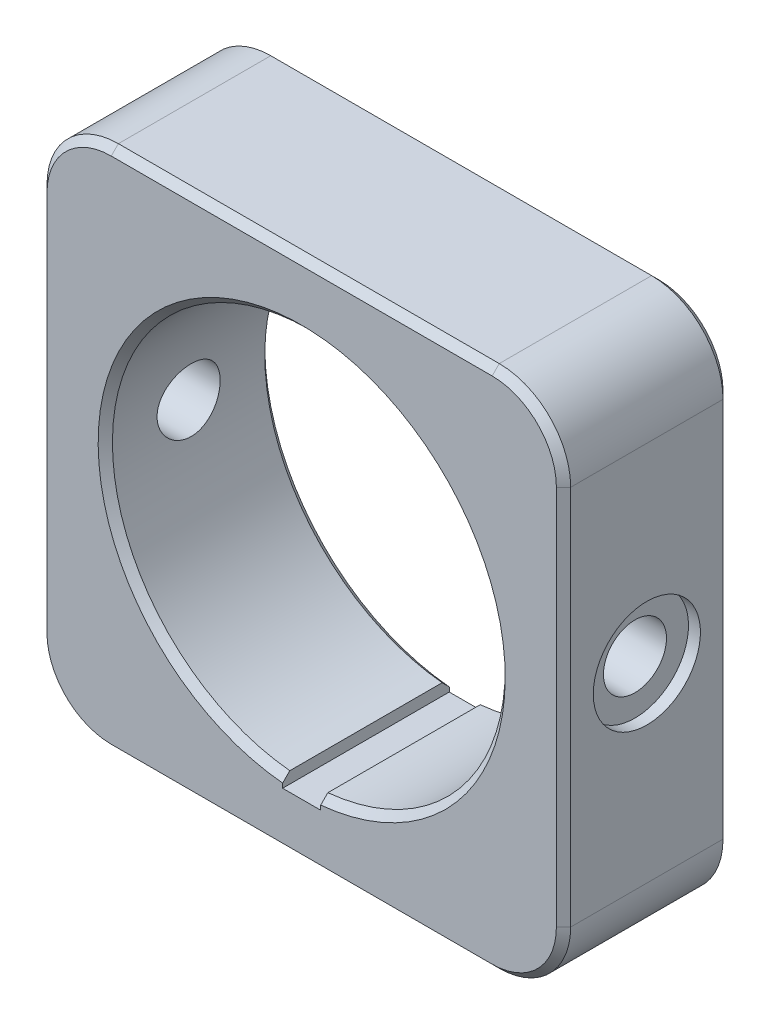
from build123d import *

# Parameters (mm, degrees)
SKETCH1_W           = 220
SKETCH1_H           = 220
BOSS_EXTRUDE1_DEPTH = 70
SKETCH2_R           = 82.5
CUT_EXTRUDE1_DEPTH  = 171.587221092
M30_TAPPED_HOLE1_D  = 26.5
SKETCH7_R           = 22.5
CUT_EXTRUDE3_DEPTH  = 5
FILLET1_R           = 30
CHAMFER1_SIZE       = 3
SKETCH8_W           = 16
SKETCH8_H           = 87
CUT_EXTRUDE4_DEPTH  = 171.587221092


with BuildPart() as part:
    # Sketch1 → Boss-Extrude1 (new body)
    with BuildSketch(Plane.XY):
        Rectangle(SKETCH1_W, SKETCH1_H)
    extrude(amount=BOSS_EXTRUDE1_DEPTH)

    # Sketch2 → Cut-Extrude1 (cut, through all)
    with BuildSketch(Plane.XY.offset(70)):
        Circle(SKETCH2_R)
    extrude(amount=-CUT_EXTRUDE1_DEPTH, mode=Mode.SUBTRACT)

    # M30 Tapped Hole1 (through all)
    with Locations(Plane(origin=(110, 0, 0), x_dir=(0, 0, -1), z_dir=(1, 0, 0))):
        with Locations((-35, 0)):
            Hole(M30_TAPPED_HOLE1_D / 2)

    # Sketch7 → Cut-Extrude3 (cut)
    with BuildSketch(Plane.ZY.offset(110)):
        with Locations((35, 0)):
            Circle(SKETCH7_R)
    cut_extrude3 = extrude(amount=-CUT_EXTRUDE3_DEPTH, mode=Mode.SUBTRACT)

    # Mirror1: Cut-Extrude3 across plane
    add(cut_extrude3.mirror(Plane(origin=(0, 0, 0), x_dir=(0, 0, 1), z_dir=(1, 0, 0))), mode=Mode.SUBTRACT)

    # Fillet1
    fillet1_edges = [part.edges().sort_by_distance(p)[0] for p in [
        (-110, 110, 35),
        (110, 110, 35),
        (110, -110, 35),
        (-110, -110, 35),
    ]]
    fillet(fillet1_edges, radius=FILLET1_R)

    # Chamfer1
    chamfer1_edges = [part.edges().sort_by_distance(p)[0] for p in [
        (-82.5, 0, 0),
        (-82.5, 0, 70),
        (0, 110, 0),
        (0, 110, 70),
        (-110, 0, 0),
        (110, 0, 0),
        (0, -110, 0),
        (-101.213203436, 101.213203436, 0),
        (-101.213203436, -101.213203436, 0),
        (101.213203436, -101.213203436, 0),
        (101.213203436, 101.213203436, 0),
        (110, 0, 70),
        (-110, 0, 70),
        (0, -110, 70),
        (-101.213203436, 101.213203436, 70),
        (-101.213203436, -101.213203436, 70),
        (101.213203436, -101.213203436, 70),
        (101.213203436, 101.213203436, 70),
    ]]
    chamfer(chamfer1_edges, length=CHAMFER1_SIZE)

    # Sketch8 → Cut-Extrude4 (cut, through all)
    with BuildSketch(Plane(origin=(0, 0, 0), x_dir=(-1, 0, 0), z_dir=(0, 0, -1))):
        with Locations((0, -43.5)):
            Rectangle(SKETCH8_W, SKETCH8_H)
    extrude(amount=-CUT_EXTRUDE4_DEPTH, mode=Mode.SUBTRACT)


solid = part.part
